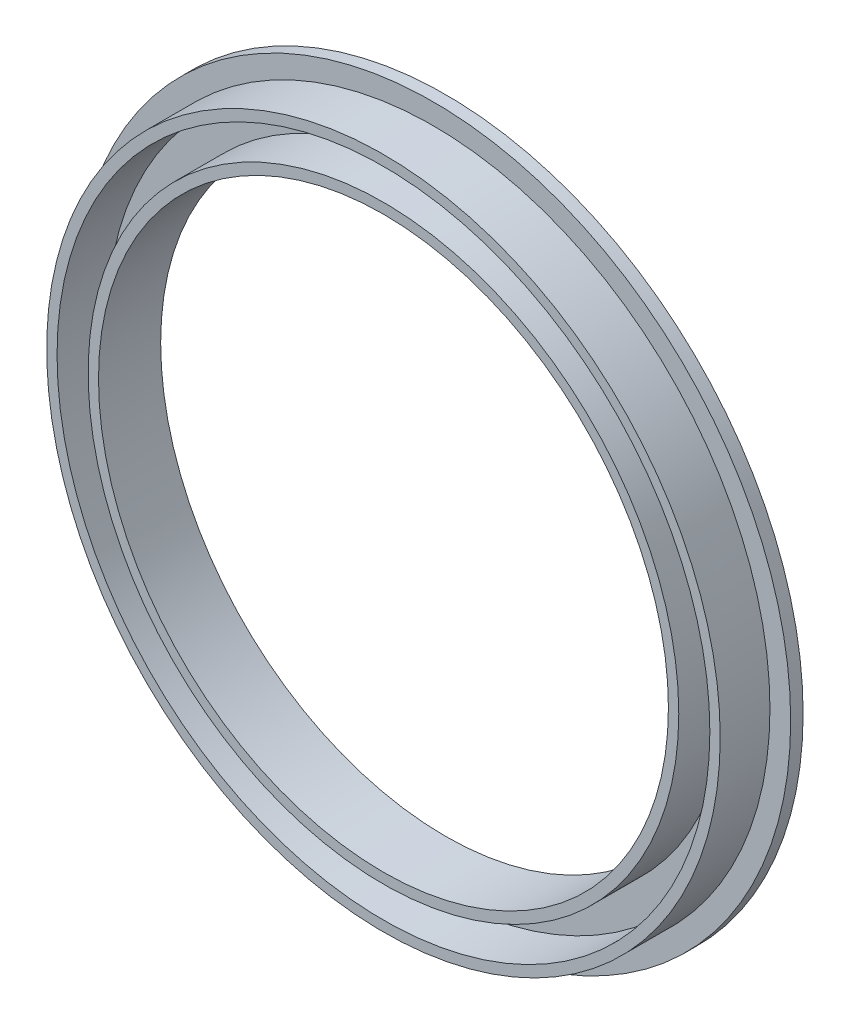
from build123d import *

# Parameters (mm, degrees)
SKETCH1_R             = 32.5
SKETCH1_R_2           = 31.5
BOSS_EXTRUDE1_DEPTH   = 6
SKETCH1_R_3           = 28.5
SKETCH1_R_4           = 27.5
BOSS_EXTRUDE1_2_DEPTH = 6
SKETCH2_R             = 34.5
SKETCH2_R_2           = 27.5
BOSS_EXTRUDE2_DEPTH   = 1.2


with BuildPart() as part:
    # Sketch1 → Boss-Extrude1 (new body)
    with BuildSketch(Plane.XY):
        Circle(SKETCH1_R)
        Circle(SKETCH1_R_2, mode=Mode.SUBTRACT)
    extrude(amount=BOSS_EXTRUDE1_DEPTH)



with BuildPart() as body_2:
    # Sketch1 → Boss-Extrude1 2 (new body)
    with BuildSketch(Plane.XY):
        Circle(SKETCH1_R_3)
        Circle(SKETCH1_R_4, mode=Mode.SUBTRACT)
    extrude(amount=BOSS_EXTRUDE1_2_DEPTH)


with BuildPart() as part_1:
    add(part.part)

    add(body_2.part)  # Boss-Extrude2 merges body 2
    # Sketch2 → Boss-Extrude2 (add)
    with BuildSketch(Plane.XY):
        Circle(SKETCH2_R)
        Circle(SKETCH2_R_2, mode=Mode.SUBTRACT)
    extrude(amount=BOSS_EXTRUDE2_DEPTH)


solid = part_1.part
